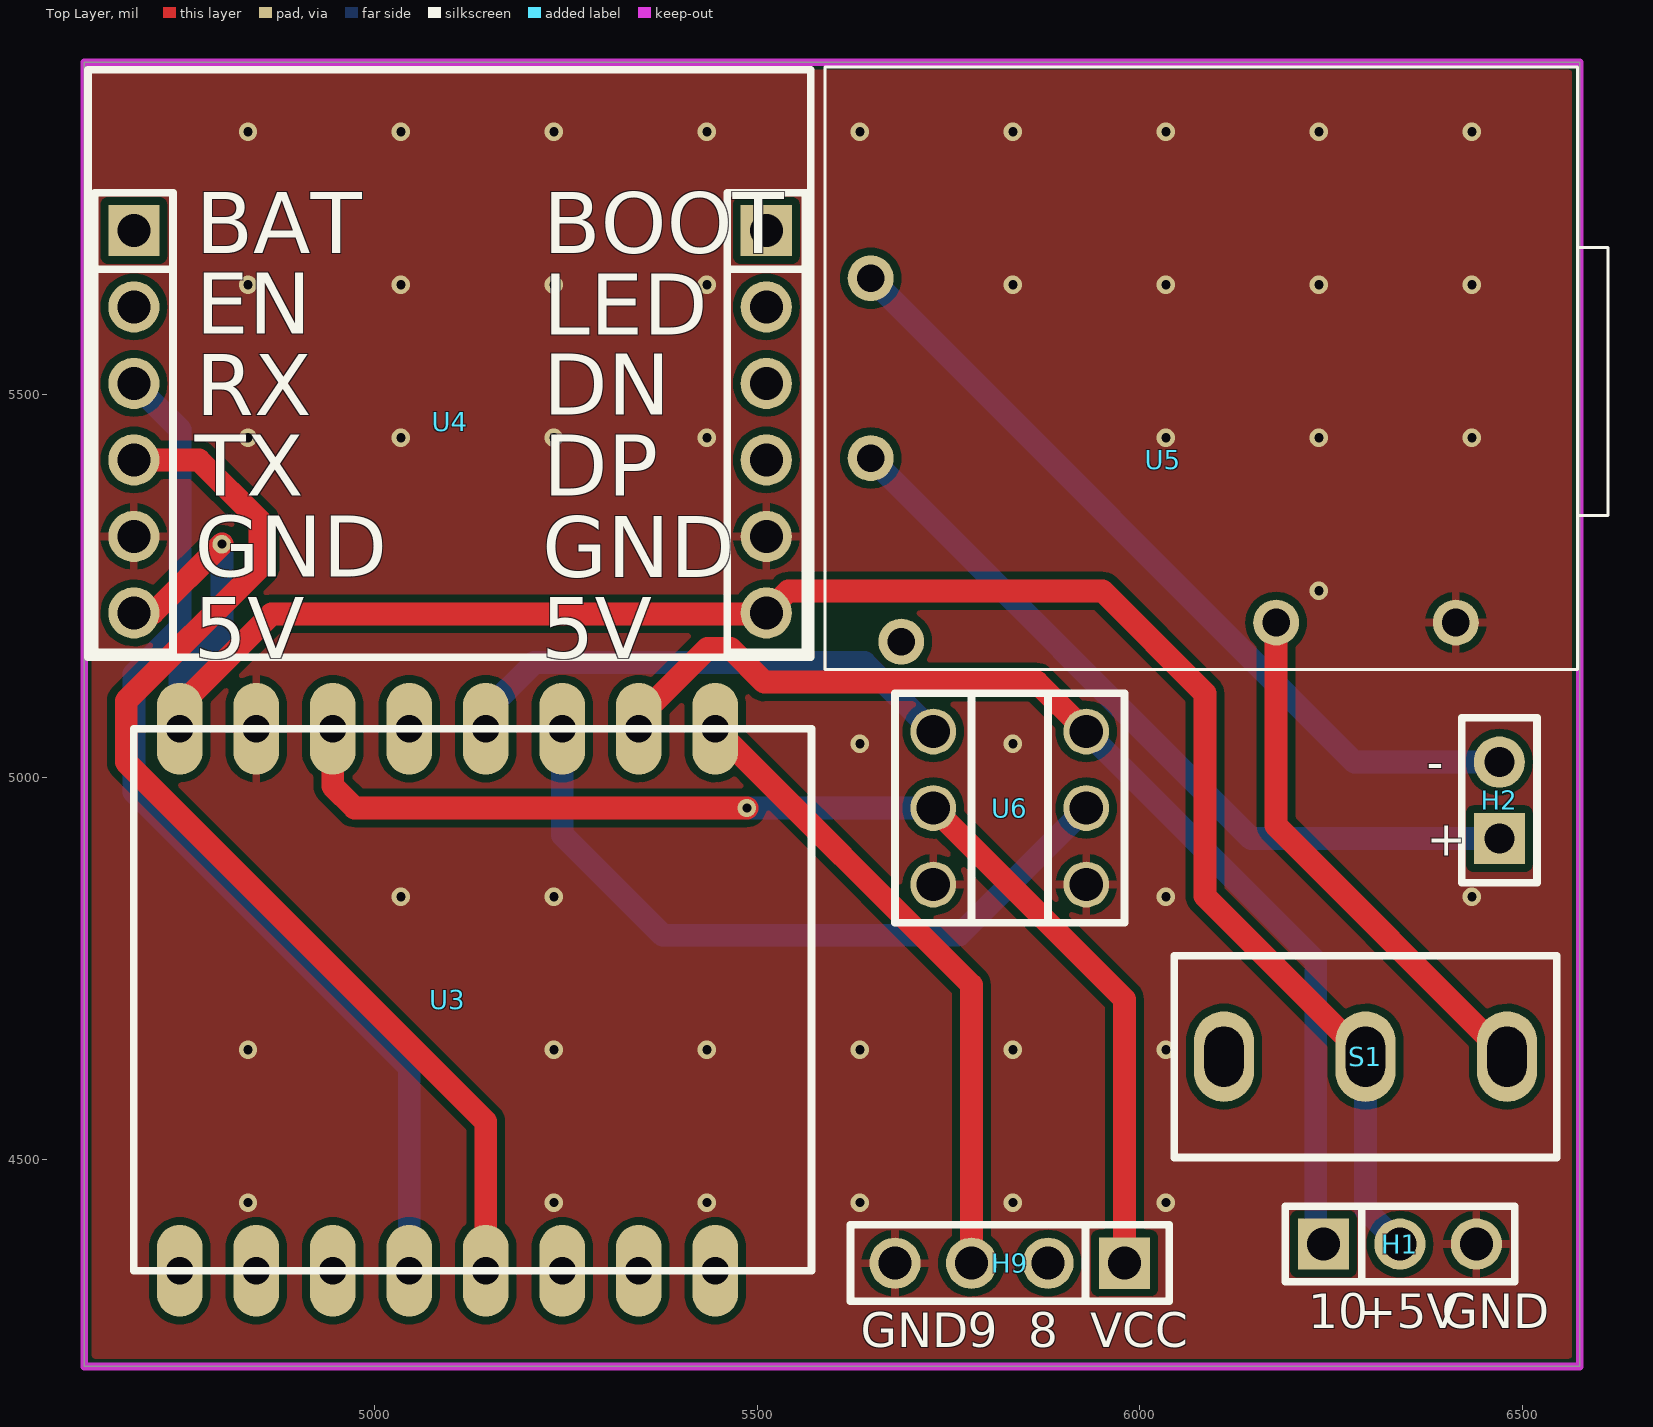
[diagram p0: Top Layer view]
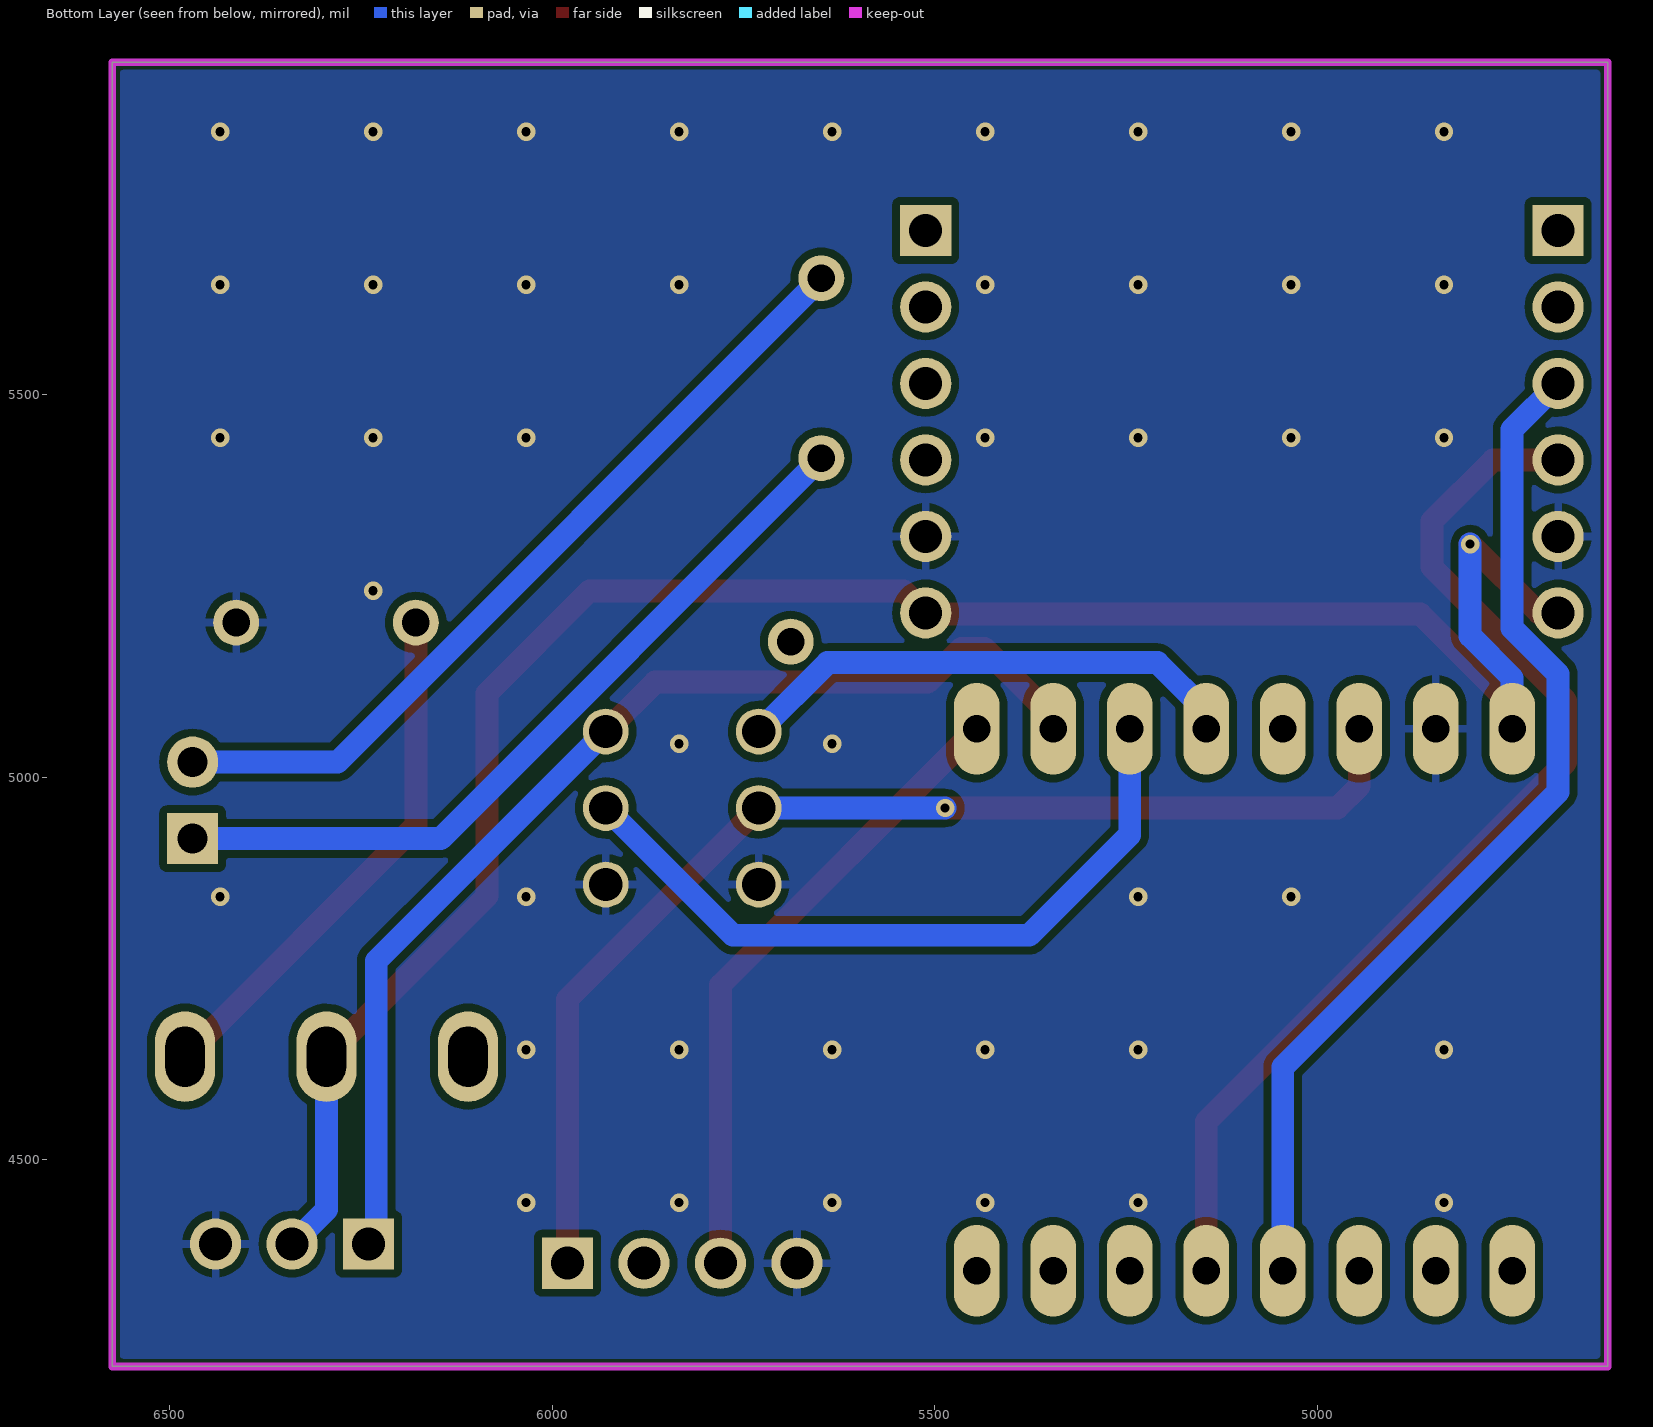
[diagram p1: Bottom Layer view, seen from below]
# Altium PCB MISC79010.pcbdoc
Units mil, origin at the board's own origin, x right, y up, seen from the top; angles counter-clockwise.
Board outline 1955 x 1705 mil, 2 copper layers (Top Layer, Bottom Layer), stack 62.206 mil thick; 8 components, 18 nets, 51 pads, 45 vias.

## Layer stack, top to bottom
Top Solder Mask Layer: solder mask 0.394, Dk 3.3
Top Layer: signal copper 1.379
Dielectric1: surface 59.449, FR4, Dk 4.5
Bottom Layer: signal copper 1.378
Bottom Solder Mask Layer: solder mask 0.394, Dk 3.3

## Board outline
4620,5935 4620,4230 6575,4230 6575,5935

## Design rules (kind name [scope] priority, off if disabled: settings)
BoardOutlineClearance copperThickness2oz_1 [All] p2 off: genericclearance=7.99 ignorepadtopadclearanceinfootprint=FALSE except(0: Arc-SplitContinuation Track-SplitContinuation SMDPad-SplitContinuation THPad-SplitContinuation Via-SplitContinuation Fill-SplitContinuation Region-SplitContinuation Poly-SplitContinuation Text-SplitContinuation Hole-SplitContinuation; 5.98: Arc-CutoutEdge Track-CutoutEdge SMDPad-CutoutEdge THPad-CutoutEdge Via-CutoutEdge Text-CutoutEdge; 6.9: Hole-OutlineEdge Hole-CutoutEdge; 10: Poly-OutlineEdge Poly-CutoutEdge; 11.81: Arc-OutlineEdge Track-OutlineEdge SMDPad-OutlineEdge THPad-OutlineEdge Via-OutlineEdge Fill-OutlineEdge Region-OutlineEdge Text-OutlineEdge Fill-CutoutEdge Region-CutoutEdge)
BoardOutlineClearance Plane_innerPlane_1 [All] p4 off: genericclearance=4.02 ignorepadtopadclearanceinfootprint=FALSE except(0: Arc-SplitContinuation Track-SplitContinuation SMDPad-SplitContinuation THPad-SplitContinuation Via-SplitContinuation Fill-SplitContinuation Region-SplitContinuation Poly-SplitContinuation Text-SplitContinuation Hole-SplitContinuation; 5.98: Arc-CutoutEdge Track-CutoutEdge SMDPad-CutoutEdge THPad-CutoutEdge Via-CutoutEdge Text-CutoutEdge; 6.9: Hole-OutlineEdge Hole-CutoutEdge; 10: Poly-OutlineEdge Poly-CutoutEdge; 11.81: Arc-OutlineEdge Track-OutlineEdge SMDPad-OutlineEdge THPad-OutlineEdge Via-OutlineEdge Fill-OutlineEdge Region-OutlineEdge Text-OutlineEdge Fill-CutoutEdge Region-CutoutEdge)
BoardOutlineClearance Copper_copperRegion_1 [All] p6 off: genericclearance=4.02 ignorepadtopadclearanceinfootprint=FALSE except(0: Arc-SplitContinuation Track-SplitContinuation SMDPad-SplitContinuation THPad-SplitContinuation Via-SplitContinuation Fill-SplitContinuation Region-SplitContinuation Poly-SplitContinuation Text-SplitContinuation Hole-SplitContinuation; 5.98: Arc-CutoutEdge Track-CutoutEdge SMDPad-CutoutEdge THPad-CutoutEdge Via-CutoutEdge Text-CutoutEdge; 6.9: Hole-OutlineEdge Hole-CutoutEdge; 10: Poly-OutlineEdge Poly-CutoutEdge; 11.81: Arc-OutlineEdge Track-OutlineEdge SMDPad-OutlineEdge THPad-OutlineEdge Via-OutlineEdge Fill-OutlineEdge Region-OutlineEdge Text-OutlineEdge Fill-CutoutEdge Region-CutoutEdge)
BoardOutlineClearance Copper_copperRegion_copperThickness1oz_1 [All] p8 off: genericclearance=4.02 ignorepadtopadclearanceinfootprint=FALSE except(0: Arc-SplitContinuation Track-SplitContinuation SMDPad-SplitContinuation THPad-SplitContinuation Via-SplitContinuation Fill-SplitContinuation Region-SplitContinuation Poly-SplitContinuation Text-SplitContinuation Hole-SplitContinuation; 5.98: Arc-CutoutEdge Track-CutoutEdge SMDPad-CutoutEdge THPad-CutoutEdge Via-CutoutEdge Text-CutoutEdge; 6.9: Hole-OutlineEdge Hole-CutoutEdge; 10: Poly-OutlineEdge Poly-CutoutEdge; 11.81: Arc-OutlineEdge Track-OutlineEdge SMDPad-OutlineEdge THPad-OutlineEdge Via-OutlineEdge Fill-OutlineEdge Region-OutlineEdge Text-OutlineEdge Fill-CutoutEdge Region-CutoutEdge)
BoardOutlineClearance Copper_copperRegion_Copper_copperRegion_1 [All] p10 off: genericclearance=4.02 ignorepadtopadclearanceinfootprint=FALSE except(0: Arc-SplitContinuation Track-SplitContinuation SMDPad-SplitContinuation THPad-SplitContinuation Via-SplitContinuation Fill-SplitContinuation Region-SplitContinuation Poly-SplitContinuation Text-SplitContinuation Hole-SplitContinuation; 5.98: Arc-CutoutEdge Track-CutoutEdge SMDPad-CutoutEdge THPad-CutoutEdge Via-CutoutEdge Text-CutoutEdge; 6.9: Hole-OutlineEdge Hole-CutoutEdge; 10: Poly-OutlineEdge Poly-CutoutEdge; 11.81: Arc-OutlineEdge Track-OutlineEdge SMDPad-OutlineEdge THPad-OutlineEdge Via-OutlineEdge Fill-OutlineEdge Region-OutlineEdge Text-OutlineEdge Fill-CutoutEdge Region-CutoutEdge)
BoardOutlineClearance copperThickness1oz_1 [All] p12: genericclearance=4.02 ignorepadtopadclearanceinfootprint=FALSE except(0: Arc-SplitContinuation Track-SplitContinuation SMDPad-SplitContinuation THPad-SplitContinuation Via-SplitContinuation Fill-SplitContinuation Region-SplitContinuation Poly-SplitContinuation Text-SplitContinuation Hole-SplitContinuation; 5.98: Arc-CutoutEdge Track-CutoutEdge SMDPad-CutoutEdge THPad-CutoutEdge Via-CutoutEdge Text-CutoutEdge; 6.9: Hole-OutlineEdge Hole-CutoutEdge; 10: Poly-OutlineEdge Poly-CutoutEdge; 11.81: Arc-OutlineEdge Track-OutlineEdge SMDPad-OutlineEdge THPad-OutlineEdge Via-OutlineEdge Fill-OutlineEdge Region-OutlineEdge Text-OutlineEdge Fill-CutoutEdge Region-CutoutEdge)
Clearance copperThickness2oz [All] p1 off: gap=7.99 ignorepadtopadclearanceinfootprint=FALSE except(5.98: SMDPad-Track SMDPad-SMDPad THPad-Track SMDPad-THPad THPad-THPad Track-Via SMDPad-Via THPad-Via Via-Via Fill-SMDPad Region-SMDPad Fill-THPad Region-THPad Fill-Via Region-Via Fill-Fill Fill-Region Region-Region Arc-Track Arc-SMDPad Arc-THPad Arc-Via Fill-Arc Region-Arc Arc-Arc Text-Track SMDPad-Text Text-THPad Text-Via Fill-Text Region-Text Arc-Text Text-Text; 6.9: Hole-Track Hole-SMDPad Hole-THPad Hole-Via Fill-Hole Region-Hole Hole-Arc Hole-Text; 10: Poly-Track Poly-SMDPad Poly-THPad Poly-Via Poly-Fill Poly-Region Poly-Poly Poly-Arc Poly-Text Poly-Hole; 11.81: Fill-Track Region-Track)
Clearance Plane_innerPlane [All] p3 off: gap=4.02 ignorepadtopadclearanceinfootprint=FALSE except(5.98: SMDPad-Track SMDPad-SMDPad THPad-Track SMDPad-THPad THPad-THPad Track-Via SMDPad-Via THPad-Via Via-Via Fill-SMDPad Region-SMDPad Fill-THPad Region-THPad Fill-Via Region-Via Fill-Fill Fill-Region Region-Region Arc-Track Arc-SMDPad Arc-THPad Arc-Via Fill-Arc Region-Arc Arc-Arc Text-Track SMDPad-Text Text-THPad Text-Via Fill-Text Region-Text Arc-Text Text-Text; 6.9: Hole-Track Hole-SMDPad Hole-THPad Hole-Via Fill-Hole Region-Hole Hole-Arc Hole-Text; 10: Poly-Track Poly-SMDPad Poly-THPad Poly-Via Poly-Fill Poly-Region Poly-Poly Poly-Arc Poly-Text Poly-Hole; 11.81: Fill-Track Region-Track)
Clearance Copper_copperRegion [All] p5 off: gap=4.02 ignorepadtopadclearanceinfootprint=FALSE except(5.98: SMDPad-Track SMDPad-SMDPad THPad-Track SMDPad-THPad THPad-THPad Track-Via SMDPad-Via THPad-Via Via-Via Fill-SMDPad Region-SMDPad Fill-THPad Region-THPad Fill-Via Region-Via Fill-Fill Fill-Region Region-Region Arc-Track Arc-SMDPad Arc-THPad Arc-Via Fill-Arc Region-Arc Arc-Arc Text-Track SMDPad-Text Text-THPad Text-Via Fill-Text Region-Text Arc-Text Text-Text; 6.9: Hole-Track Hole-SMDPad Hole-THPad Hole-Via Fill-Hole Region-Hole Hole-Arc Hole-Text; 10: Poly-Track Poly-SMDPad Poly-THPad Poly-Via Poly-Fill Poly-Region Poly-Poly Poly-Arc Poly-Text Poly-Hole; 11.81: Fill-Track Region-Track)
Clearance Copper_copperRegion_copperThickness1oz [All] p7 off: gap=4.02 ignorepadtopadclearanceinfootprint=FALSE except(5.98: SMDPad-Track SMDPad-SMDPad THPad-Track SMDPad-THPad THPad-THPad Track-Via SMDPad-Via THPad-Via Via-Via Fill-SMDPad Region-SMDPad Fill-THPad Region-THPad Fill-Via Region-Via Fill-Fill Fill-Region Region-Region Arc-Track Arc-SMDPad Arc-THPad Arc-Via Fill-Arc Region-Arc Arc-Arc Text-Track SMDPad-Text Text-THPad Text-Via Fill-Text Region-Text Arc-Text Text-Text; 6.9: Hole-Track Hole-SMDPad Hole-THPad Hole-Via Fill-Hole Region-Hole Hole-Arc Hole-Text; 10: Poly-Track Poly-SMDPad Poly-THPad Poly-Via Poly-Fill Poly-Region Poly-Poly Poly-Arc Poly-Text Poly-Hole; 11.81: Fill-Track Region-Track)
Clearance Copper_copperRegion_Copper_copperRegion [All] p9 off: gap=4.02 ignorepadtopadclearanceinfootprint=FALSE except(5.98: SMDPad-Track SMDPad-SMDPad THPad-Track SMDPad-THPad THPad-THPad Track-Via SMDPad-Via THPad-Via Via-Via Fill-SMDPad Region-SMDPad Fill-THPad Region-THPad Fill-Via Region-Via Fill-Fill Fill-Region Region-Region Arc-Track Arc-SMDPad Arc-THPad Arc-Via Fill-Arc Region-Arc Arc-Arc Text-Track SMDPad-Text Text-THPad Text-Via Fill-Text Region-Text Arc-Text Text-Text; 6.9: Hole-Track Hole-SMDPad Hole-THPad Hole-Via Fill-Hole Region-Hole Hole-Arc Hole-Text; 10: Poly-Track Poly-SMDPad Poly-THPad Poly-Via Poly-Fill Poly-Region Poly-Poly Poly-Arc Poly-Text Poly-Hole; 11.81: Fill-Track Region-Track)
Clearance copperThickness1oz [All] p11: gap=4.02 ignorepadtopadclearanceinfootprint=FALSE except(5.98: SMDPad-Track SMDPad-SMDPad THPad-Track SMDPad-THPad THPad-THPad Track-Via SMDPad-Via THPad-Via Via-Via Fill-SMDPad Region-SMDPad Fill-THPad Region-THPad Fill-Via Region-Via Fill-Fill Fill-Region Region-Region Arc-Track Arc-SMDPad Arc-THPad Arc-Via Fill-Arc Region-Arc Arc-Arc Text-Track SMDPad-Text Text-THPad Text-Via Fill-Text Region-Text Arc-Text Text-Text; 6.9: Hole-Track Hole-SMDPad Hole-THPad Hole-Via Fill-Hole Region-Hole Hole-Arc Hole-Text; 10: Poly-Track Poly-SMDPad Poly-THPad Poly-Via Poly-Fill Poly-Region Poly-Poly Poly-Arc Poly-Text Poly-Hole; 11.81: Fill-Track Region-Track)
DiffPairsRouting differentialPair [All] p1: maxlimit=6 minlimit=6 mostfreqgap=6 toplayer_minwidth=5 toplayer_prefwidth=10 toplayer_maxwidth=100 toplayer_mingap=6 toplayer_prefgap=6 toplayer_maxgap=6 bottomlayer_minwidth=5 bottomlayer_prefwidth=10 bottomlayer_maxwidth=100 bottomlayer_mingap=6 bottomlayer_prefgap=6 bottomlayer_maxgap=6 maxuncoupledlength=10
HoleToHoleClearance otherClearance [All] p1: gap=11.81 allowstackedmicrovias=TRUE
Length netLength [All] p1: minlimit=0 maxlimit=0
MatchedLengths netLengthTolerance [All] p1: tolerance=1000
PasteMaskExpansion pasteMaskExpansion [All] p1: expansion=0
PlaneConnect innerPlane [All] p1: planeconnectstyle=Relief reliefexpansion=20 reliefentries=4 reliefconductorwidth=10 reliefairgap=10
PolygonConnect copperRegion_copperThickness1oz [(InNet('GND'))] p1: connectstyle=Relief reliefconductorwidth=10 reliefentries=4 polygonreliefangle="90 Angle" airgapwidth=10 via.connectstyle=Relief via.reliefconductorwidth=10 via.reliefentries=4 via.polygonreliefangle="90 Angle" via.airgapwidth=10
PolygonConnect copperRegion_Copper_copperRegion [All] p2 off: connectstyle=Relief reliefconductorwidth=10 reliefentries=4 polygonreliefangle="90 Angle" airgapwidth=10 via.connectstyle=Relief via.reliefconductorwidth=10 via.reliefentries=4 via.polygonreliefangle="90 Angle" via.airgapwidth=10
PolygonConnect copperRegion [All] p3: connectstyle=Relief reliefconductorwidth=10 reliefentries=4 polygonreliefangle="90 Angle" airgapwidth=10 via.connectstyle=Relief via.reliefconductorwidth=10 via.reliefentries=4 via.polygonreliefangle="90 Angle" via.airgapwidth=10
RoutingVias viaSize [All] p1: holewidth=12.01 width=24.02 viastyle="Through Hole" minholewidth=11.81 minwidth=19.68 maxholewidth=248.03 maxwidth=393.7
SolderMaskExpansion solderMaskExpansion [IsVia] p1: expansion=-1000 istentingtop=TRUE
SolderMaskExpansion solderMaskExpansion [All] p2: expansion=2 istentingtop=FALSE
Width copperThickness2oz_2 [All] p1 off: maxlimit=100 minlimit=8 preferedwidth=10
Width copperThickness1oz_2 [All] p2: maxlimit=10 minlimit=10 preferedwidth=10 toplayer_minwidth=30 toplayer_maxwidth=100 toplayer_prefwidth=30 bottomlayer_minwidth=30 bottomlayer_maxwidth=100 bottomlayer_prefwidth=30

## Components (designator, comment, footprint, x,y, rotation, side; value= is the part's Value field where it differs from the comment)
H1 "" HDR-TH_3P-P2.54-V-M 6340,4390 r0 top
H2 "" HDR-TH_2P-P2.54-V-F 6470,4970 r90 top
H9 "" HDR-TH_4P-P2.54-V-F 5830,4365 r180 top
S1 "SS-12D10L5" SS-12D10L5 6295,4635 r0 top
U3 "" 【封装Supermini】 5185,4705 r90 top
U4 "" ML307C-GC核心板 5100,5560 r0 top
U5 "" 5V2A充放电一体模块 6100,5535 r90 top
U6 "INMP441" INMP441 5830,4960 r0 top

## Footprints (in the part's own frame and the unit in brackets; to place one, negate y for a bottom-side part, rotate by r counter-clockwise, add the part's x,y. Pads: shape width x height; smd on the part's side, far side on the other; paste and mask are expansions set on the pad)
5V2A充放电一体模块 [mil]
  round 60 hole 36 paste+0 mask+2: 1(-117.54,451.82) 2(117.5,451.82) 3(-332.52,-313.18) 4(-332.52,-78.18) 5(-357.52,411.82)
  silkscreen extent -394,-512 394,512
HDR-TH_2P-P2.54-V-F [mm]
  rect 1.7x1.7 hole 1: 1(-1.27,0)
  round 1.7 hole 1: 2(1.27,0)
  silkscreen extent -2.74,-1.25 2.74,1.25
HDR-TH_3P-P2.54-V-M [mm]
  rect 1.7x1.7 hole 1.1: 1(-2.54,0)
  round 1.7 hole 1.1: 2(0,0) 3(2.54,0)
  silkscreen extent -3.81,-1.25 3.81,1.25
HDR-TH_4P-P2.54-V-F [mm]
  rect 1.7x1.7 hole 1.1: 1(-3.81,0)
  round 1.7 hole 1.1: 2(-1.27,0) 3(1.27,0) 4(3.81,0)
  silkscreen extent -5.29,-1.27 5.29,1.27
INMP441 [mil]
  round 60 hole 43.31: 1(-100,100) 2(-100,0) 3(-100,-100) 4(100,-100) 5(100,0) 6(100,100)
  silkscreen extent -150,-150 150,150
ML307C-GC核心板 [mm]
  rect 1.7x1.7 hole 1.1: 1(-10.541,3.937) 12(10.459,3.937)
  round 1.7 hole 1.1: 2(-10.541,1.397) 3(-10.541,-1.143) 4(-10.541,-3.683) 5(-10.541,-6.223) 6(-10.541,-8.763) 7(10.459,-8.763) 8(10.459,-6.223) 9(10.459,-3.683) 10(10.459,-1.143) 11(10.459,1.397)
  silkscreen extent -12.06,-10.23 11.94,9.27
SS-12D10L5 [mm]
  oval 2x3 hole 1.3 slot 2 at 90 deg: 1(-4.7,0) 2(0,0) 3(4.7,0)
  silkscreen extent -6.35,-3.35 6.35,3.35
【封装Supermini】 [mil]
  oval 120x60 hole 36: 1(-350,440) 2(-350,340) 3(-350,240) 4(-350,140) 5(-350,40) 6(-350,-60) 7(-350,-160) 8(-350,-260) 9(358.66,-260) 10(358.66,-160) 11(358.66,-60) 12(358.66,40) 13(358.66,140) 14(358.66,240) 15(358.66,340) 16(358.66,440)
  silkscreen extent -350,-386 359,500

## Via types
v1: diameter 24.02, hole 12, Top Layer to Bottom Layer, 45 vias

## Nets (pads, with @x,y where several pads share a name; then routed paths per layer and width w, separated by ;. In a path a pad name is that pad's centre, name@x,y a point inside that pad or via, vN(x,y) a via of type N, cw(c..) or ccw(c..) an arc to the next point about the centre after c; other vN are vias at no path point)
1: U3.1
2: U3.2
3: U3.3
4: U3.4 U4.3 | length 1358.8
  Bottom Layer w30: U4.3 4745,5455 4745,5195 4685,5135 4685,4981.22 5045,4621.22 U3.4
5: U3.5 U4.4 | length 1445.3
  Top Layer w30: U4.4 4770,5415 4850,5335 4850,5275 4675,5100 4675,5020 5145,4550 U3.5
6: U3.6
8: H9.2
9: H9.3 U3.9 | length 837.4
  Top Layer w30: U3.9 5780,4728.66 H9.3
10: H1.1 U3.10 U6.6 | length 1480.7
  Top Layer w30: U3.10 5345,5078.66 5435,5168.66 5465,5168.66 5509.06,5124.6 5865.39,5124.6 U6.6
  Bottom Layer w30: U6.6 6230,4760 6230,4400 H1.1
11: U3.11 U6.5 | length 947
  Bottom Layer w30: U3.11 5245,4925 5376.34,4793.66 5763.66,4793.66 U6.5
12: U3.12 U6.1 | length 671.3
  Bottom Layer w30: U3.12 5145,5086.34 5208.66,5150 5640,5150 U6.1
13: U3.13
$1N17589: H2.1 U5.1 | length 1027.9
  Bottom Layer w30: U5.1 6145.65,4920 H2.1
$1N17590: H2.2 U5.2 | length 1083.8
  Bottom Layer w30: U5.2 6280.68,5020 H2.2
$1N17591: S1.3 U5.4 | length 692.5
  Top Layer w30: U5.4 6178.18,4936.86 S1.3
+5V: H1.2 S1.2 U3.16 U4.6 U4.7 | length 2729.5
  Top Layer w30: U4.6 4710,5215 v1(4800,5305) ; U3.16 4745,5093.66 4865,5213.66 5510.43,5213.66 5540.43,5243.66 5951.34,5243.66 6085,5110 6085,4845 S1.2
  Bottom Layer w30: U3.16 4745,5130 4800,5185 v1(4800,5305) ; S1.2 6295,4435 H1.2
GND: H1.3 H9.4 U3.15 U4.5 U4.8 U5.3 U6.3 U6.4
  other v1: 4834.1,4444.1 5234.1,4444.1 5434.1,4444.1 5634.1,4444.1 5834.1,4444.1 6034.1,4444.1 4834.1,4644.1 5234.1,4644.1 5434.1,4644.1 5634.1,4644.1 5834.1,4644.1 6034.1,4644.1 5034.1,4844.1 5234.1,4844.1 6034.1,4844.1 6434.1,4844.1 5634.1,5044.1 5834.1,5044.1 6234.1,5244.1 4834.1,5444.1 5034.1,5444.1 5234.1,5444.1 5434.1,5444.1 6034.1,5444.1 6234.1,5444.1 6434.1,5444.1 4834.1,5644.1 5034.1,5644.1 5234.1,5644.1 5434.1,5644.1 5834.1,5644.1 6034.1,5644.1 6234.1,5644.1 6434.1,5644.1 4834.1,5844.1 5034.1,5844.1 5234.1,5844.1 5434.1,5844.1 5634.1,5844.1 5834.1,5844.1 6034.1,5844.1 6234.1,5844.1 6434.1,5844.1
VCC: H9.1 U3.14 U6.2 | length 1570.4
  Top Layer w30: U3.14 4945,4988.66 4973.66,4960 v1(5486.34,4960) ; U6.2 5980,4710 H9.1
  Bottom Layer w30: v1(5486.34,4960) U6.2
pads on no net: S1.1 U3.7 U3.8 U4.1 U4.2 U4.9 U4.10 U4.11 U4.12 U5.5

## Polygon pours and split planes (outlines as drawn)
GND on Top Layer (solid, remove dead copper, pour order 0): 3705,6715 3705,3000 7375,3000 7375,6715
GND on Bottom Layer (solid, remove dead copper, pour order 2): 3600,6580 3600,3145 7515,3145 7515,6580

## Keep-outs
Board Outline Layer:
  the board outline again, w10

## Silkscreen, mask and mechanical layers (free items; w line width, h text height)
Top Silkscreen Layer:
  lines w10: 5680,4810 5680,5110 5980,5110 5980,4810 5680,4810
  text "-" at 6374.86,4997.5 h45
  text "+" at 6374.86,4897.5 h45
  text "10" at 6220,4280 h45
  text "+5V" at 6283.9,4280 h45
  text "GND" at 6395,4280 h45
  text "GND" at 5635,4255 h45
  text "9" at 5774.77,4255 h45
  text "8" at 5854.23,4255 h45
  text "VCC" at 5935,4255 h45